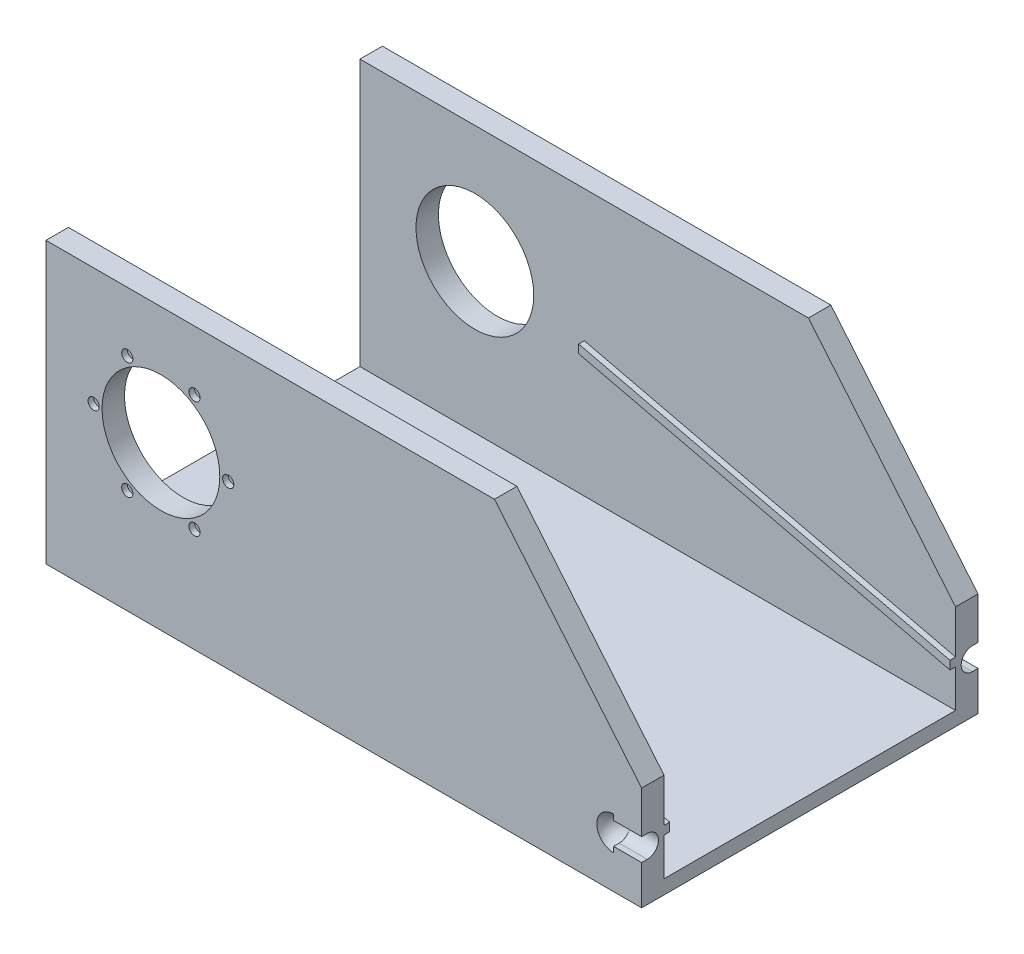
from build123d import *

# Parameters (mm, degrees)
EXTRUDE_1_DEPTH          = 80
SKETCH_4_W               = 520
SKETCH_4_H               = 50
EXTRUDE_2_DEPTH          = 2125
EXTRUDE_3_DEPTH          = 80
CUT_EXTRUDE_3_DEPTH      = 2638.351891576
CUT_EXTRUDE_3_DEPTH_BACK = 2638.351891576
SKETCH_2_R               = 210
EXTRUDE_4_DEPTH          = 100
SKETCH_7_R               = 20
CUT_EXTRUDE_5_DEPTH      = 20
CUT_EXTRUDE_6_DEPTH      = 100
CUT_REVOLVE_1_ANGLE      = 90


with BuildPart() as part:
    # 草图1 → 凸台-拉伸1 (new body)
    with BuildSketch(Plane.XY):
        Polygon((0, 0), (0, -1000), (2125, -1000), (2125, -630), (1600, 0), align=None)
    extrude(amount=EXTRUDE_1_DEPTH)

    # 草图4 → 凸台-拉伸2 (add)
    with BuildSketch(Plane(origin=(0, 0, 0), x_dir=(0, 0, -1), z_dir=(1, 0, 0))):
        with Locations((-340, -975)):
            Rectangle(SKETCH_4_W, SKETCH_4_H)
    extrude_2 = extrude(amount=EXTRUDE_2_DEPTH)

    # 镜向4: 凸台-拉伸2 across plane
    add(extrude_2.mirror(Plane.XY.offset(600)))

    # 草图5 → 凸台-拉伸3 (add)
    with BuildSketch(Plane.XY.offset(1120)):
        Polygon((0, -1000), (0, 0), (1600, 0), (2125, -630), (2125, -1000), align=None)
    extrude(amount=EXTRUDE_3_DEPTH)

    # 草图2 → 切除-拉伸3 (cut, two sides: drawn at the far end of the back side and taken through both)
    with BuildSketch(Plane.XY.offset(-CUT_EXTRUDE_3_DEPTH_BACK)):
        with Locations(Location((410, -420, 0), (0, 0, 180))):
            Circle(SKETCH_2_R)
    extrude(amount=CUT_EXTRUDE_3_DEPTH + CUT_EXTRUDE_3_DEPTH_BACK, mode=Mode.SUBTRACT)

    # 草图6 → 凸台-拉伸4 (add)
    with BuildSketch(Plane.XY):
        Polygon((800.5, -500), (2125, -815), (2125, -785), (800.5, -470), align=None)
    extrude_4 = extrude(amount=EXTRUDE_4_DEPTH)

    # 镜向5: 凸台-拉伸4 across plane
    add(extrude_4.mirror(Plane.XY.offset(600)))

    # 草图7 → 切除-拉伸5 (cut)
    with BuildSketch(Plane.XY):
        with Locations((170, -420)):
            Circle(SKETCH_7_R)
        with Locations((289.999999999, -627.846096908)):
            Circle(SKETCH_7_R)
        with Locations((530.000000001, -627.846096908)):
            Circle(SKETCH_7_R)
        with Locations((650, -420)):
            Circle(SKETCH_7_R)
        with Locations((289.999999999, -212.153903092)):
            Circle(SKETCH_7_R)
        with Locations((530.000000001, -212.153903092)):
            Circle(SKETCH_7_R)
    cut_extrude_5 = extrude(amount=CUT_EXTRUDE_5_DEPTH, mode=Mode.SUBTRACT)

    # 镜向6: 切除-拉伸5 across plane
    add(cut_extrude_5.mirror(Plane.XY.offset(600)), mode=Mode.SUBTRACT)

    # 草图8 → 切除-拉伸6 (cut)
    with BuildSketch(Plane(origin=(2125, 0, 0), x_dir=(0, 0, -1), z_dir=(1, 0, 0))):
        with BuildLine():
            Line((-1200, -860), (-1180, -860))
            ThreePointArc((-1180, -860), (-1140, -820), (-1180, -780))
            Line((-1180, -780), (-1200, -780))
            Line((-1200, -780), (-1200, -860))
        make_face()
    cut_extrude_6 = extrude(amount=-CUT_EXTRUDE_6_DEPTH, mode=Mode.SUBTRACT)

    # 草图9 → 切除-旋转1 (revolve, cut)
    with BuildSketch(Plane.XY.offset(1200)):
        with BuildLine():
            Line((2025, -760), (2025, -880))
            ThreePointArc((2025, -880), (1965, -820), (2025, -760))
        make_face()
    cut_revolve_1 = revolve(axis=Axis((2025, -760, 1200), (0, -1, 0)), revolution_arc=CUT_REVOLVE_1_ANGLE, mode=Mode.SUBTRACT)

    # 镜向7: 切除-拉伸6, 切除-旋转1 across plane
    add(cut_extrude_6.mirror(Plane.XY.offset(600)), mode=Mode.SUBTRACT)
    add(cut_revolve_1.mirror(Plane.XY.offset(600)), mode=Mode.SUBTRACT)


solid = part.part
